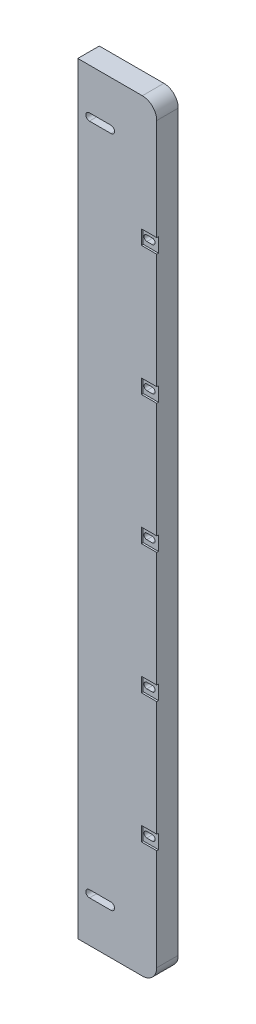
from build123d import *

# Parameters (mm, degrees)
SKETCH_1_W             = 44
SKETCH_1_H             = 425
EXTRUDE_1_DEPTH        = 12
FILLET_1_R             = 8
CUT_EXTRUDE_1_DEPTH    = 6
CUT_EXTRUDE_2_DEPTH    = 214.720027138
SKETCH_6_W             = 8.5
SKETCH_6_H             = 8
CUT_EXTRUDE_4_DEPTH    = 1
CUT_EXTRUDE_5_DEPTH    = 4
CUT_EXTRUDE_6_DEPTH    = 214.785523364
PATTERN_LINEAR_1_COUNT = 5
PATTERN_LINEAR_1_PITCH = 72


with BuildPart() as part:
    # 草图1 → 凸台-拉伸1 (new body)
    with BuildSketch(Plane.XY):
        Rectangle(SKETCH_1_W, SKETCH_1_H)
    extrude(amount=EXTRUDE_1_DEPTH)

    # 圆角1
    fillet_1_edges = [part.edges().sort_by_distance(p)[0] for p in [
        (22, 212.5, 6),
        (22, -212.5, 6),
    ]]
    fillet(fillet_1_edges, radius=FILLET_1_R)

    # 草图3 → 切除-拉伸1 (cut)
    with BuildSketch(Plane(origin=(0, 0, 0), x_dir=(-1, 0, 0), z_dir=(0, 0, -1))):
        with BuildLine():
            Line((3.5, 191.5), (15.5, 191.5))
            ThreePointArc((15.5, 191.5), (19.5, 187.5), (15.5, 183.5))
            Line((15.5, 183.5), (3.5, 183.5))
            ThreePointArc((3.5, 183.5), (-0.5, 187.5), (3.5, 191.5))
        make_face()
        with BuildLine():
            Line((3.5, -191.5), (15.5, -191.5))
            ThreePointArc((15.5, -191.5), (19.5, -187.5), (15.5, -183.5))
            Line((15.5, -183.5), (3.5, -183.5))
            ThreePointArc((3.5, -183.5), (-0.5, -187.5), (3.5, -191.5))
        make_face()
    extrude(amount=-CUT_EXTRUDE_1_DEPTH, mode=Mode.SUBTRACT)

    # 草图4 → 切除-拉伸2 (cut, through all)
    with BuildSketch(Plane(origin=(0, 0, 6), x_dir=(-1, 0, 0), z_dir=(0, 0, -1))):
        with BuildLine():
            Line((3.5, 189.5), (15.5, 189.5))
            ThreePointArc((15.5, 189.5), (17.5, 187.5), (15.5, 185.5))
            Line((15.5, 185.5), (3.5, 185.5))
            ThreePointArc((3.5, 185.5), (1.5, 187.5), (3.5, 189.5))
        make_face()
        with BuildLine():
            Line((3.5, -189.5), (15.5, -189.5))
            ThreePointArc((15.5, -189.5), (17.5, -187.5), (15.5, -185.5))
            Line((15.5, -185.5), (3.5, -185.5))
            ThreePointArc((3.5, -185.5), (1.5, -187.5), (3.5, -189.5))
        make_face()
    extrude(amount=-CUT_EXTRUDE_2_DEPTH, mode=Mode.SUBTRACT)

    # 草图6 → 切除-拉伸4 (cut)
    with BuildSketch(Plane.XY.offset(12)):
        with Locations((17.75, 144)):
            Rectangle(SKETCH_6_W, SKETCH_6_H)
        with Locations((17.75, 72)):
            Rectangle(SKETCH_6_W, SKETCH_6_H)
        with Locations((17.75, 0)):
            Rectangle(SKETCH_6_W, SKETCH_6_H)
        with Locations((17.75, -72)):
            Rectangle(SKETCH_6_W, SKETCH_6_H)
        with Locations((17.75, -144)):
            Rectangle(SKETCH_6_W, SKETCH_6_H)
    extrude(amount=-CUT_EXTRUDE_4_DEPTH, mode=Mode.SUBTRACT)

    # 草图7 → 切除-拉伸5 (cut)
    with BuildSketch(Plane(origin=(0, 0, 0), x_dir=(-1, 0, 0), z_dir=(0, 0, -1))):
        with BuildLine():
            Line((-18.5, 147), (-15.5, 147))
            ThreePointArc((-15.5, 147), (-12.5, 144), (-15.5, 141))
            Line((-15.5, 141), (-18.5, 141))
            ThreePointArc((-18.5, 141), (-21.5, 144), (-18.5, 147))
        make_face()
    cut_extrude_5 = extrude(amount=-CUT_EXTRUDE_5_DEPTH, mode=Mode.SUBTRACT)

    # 草图8 → 切除-拉伸6 (cut, through all)
    with BuildSketch(Plane(origin=(0, 0, 4), x_dir=(-1, 0, 0), z_dir=(0, 0, -1))):
        with BuildLine():
            Line((-18.5, 145.6), (-15.5, 145.6))
            ThreePointArc((-15.5, 145.6), (-13.9, 144), (-15.5, 142.4))
            Line((-15.5, 142.4), (-18.5, 142.4))
            ThreePointArc((-18.5, 142.4), (-20.1, 144), (-18.5, 145.6))
        make_face()
    cut_extrude_6 = extrude(amount=-CUT_EXTRUDE_6_DEPTH, mode=Mode.SUBTRACT)

    # 阵列(线性)1: 切除-拉伸5, 切除-拉伸6 ×5
    with Locations(*[(0, -i * PATTERN_LINEAR_1_PITCH, 0) for i in range(1, PATTERN_LINEAR_1_COUNT)]):
        add(cut_extrude_5, mode=Mode.SUBTRACT)
        add(cut_extrude_6, mode=Mode.SUBTRACT)


solid = part.part
